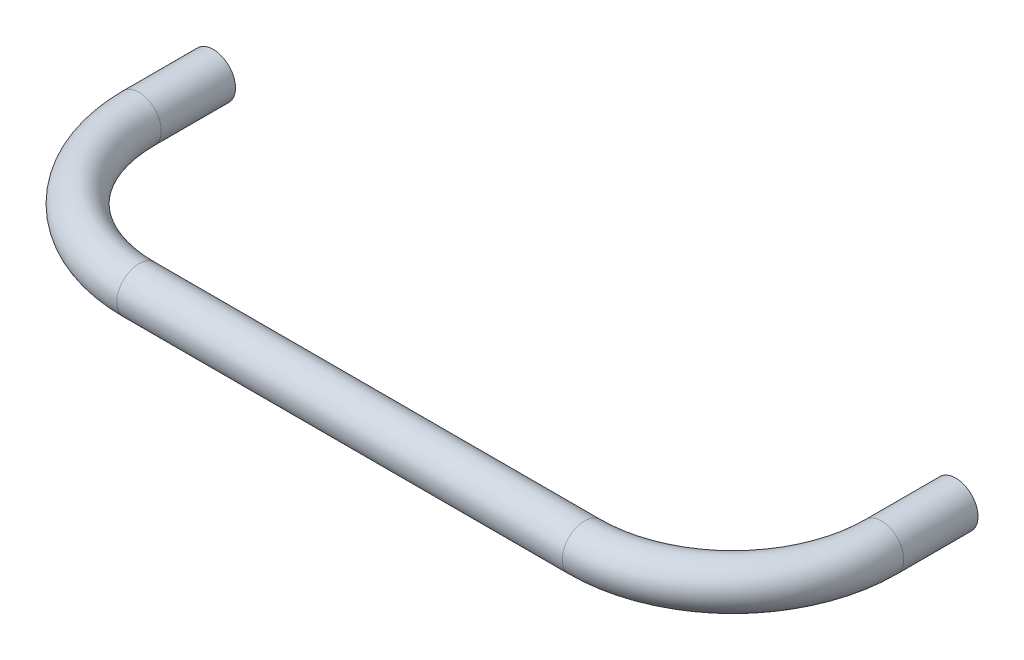
SolidWorks part; units mm, degrees
ref_plane "Front Plane" through (0, 0, 0) normal (0, 0, 1) x (1, 0, 0)
ref_plane "Top Plane" through (0, 0, 0) normal (0, 1, 0) x (1, 0, 0)
ref_plane "Right Plane" through (0, 0, 0) normal (1, 0, 0) x (0, 0, -1)
sketch "Sketch1" plane through (0, 0, 0) normal (0, 1, 0) x (1, 0, 0)
  line L0 (100, 0) -> (400, 0)
  line L1 (500, 100) -> (500, 150)
  line L2 (0, 100) -> (0, 150)
  arc A0 (400, 0) -> (500, 100) centre (400, 100) ccw
  arc A1 (100, 0) -> (0, 100) centre (100, 100) cw
  point P7 (500, 0)
  point P10 (0, 0)
  dimension "D4" = 100
  dimension "D1" = 500
  dimension "D2" = 150
  dimension "D3" = 150
sweep "Sweep1" add path "Sketch1" circular profile diameter 30 parameters "D3"=30
hole_wizard "M10 Tapped Hole1" positions "Sketch16" profile "Sketch18" tap size "M10" standard "GB"
sketch "Sketch16" plane through (0, 0, -150) normal (0, 0, -1) x (-1, 0, 0)
  point P0 (-500, 0)
  point P3 (0, 0)
sketch "Sketch18" plane through (500, 0, -150) normal (1, 0, 0) x (0, 1, 0)
  line L0 (0, 0) -> (0, 34.0537)
  line L1 (0, 34.0537) -> (4.25, 31.5)
  line L2 (4.25, 31.5) -> (4.25, 0)
  line L5 (4.25, 0) -> (0, 0)
  line L10 (0, 34.0537) -> (-4.25, 31.5) construction
  line L11 (0, -6.35) -> (0, 107.95) construction
  dimension "螺纹孔钻头直径" = 8.5
  dimension "螺纹孔钻头深度" = 31.5
  dimension "导头角度" = 118
cosmetic thread "Hole Thread1" parameters "D1"=24, "D2"=10
cosmetic thread "Hole Thread2" parameters "D1"=24, "D2"=10
